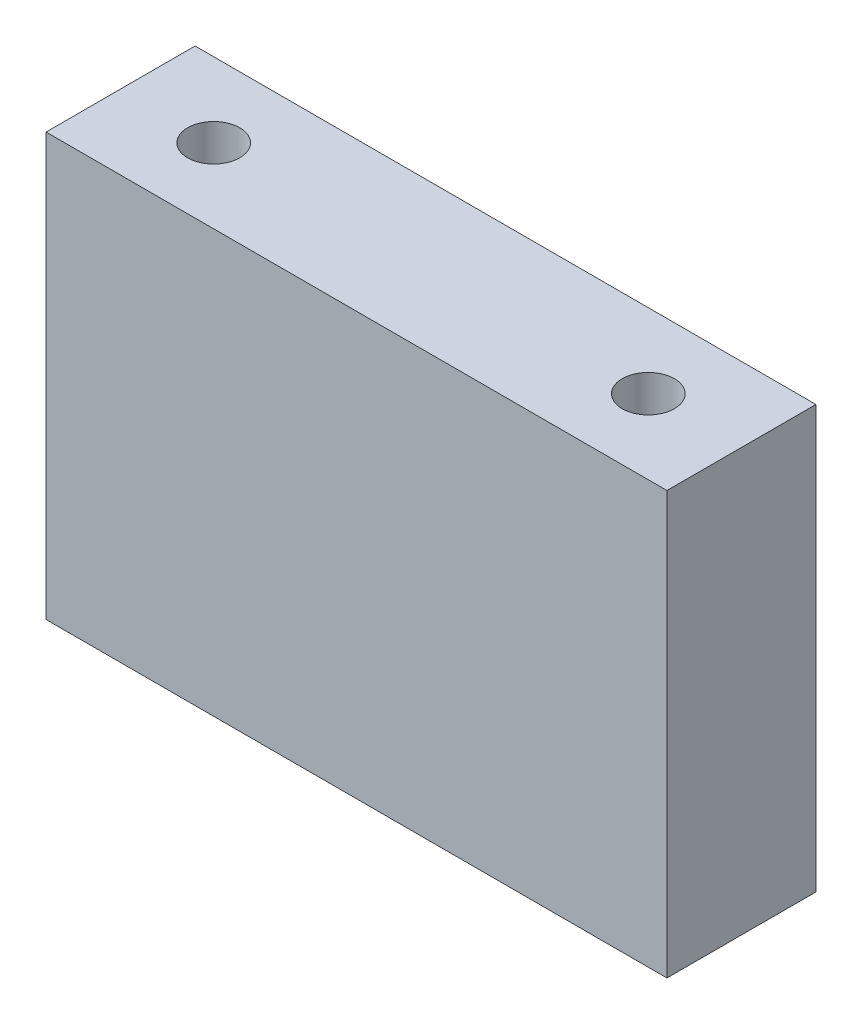
from build123d import *

# Parameters (mm, degrees)
SKETCH_1_W                  = 50
SKETCH_1_H                  = 34
EXTRUDE_1_DEPTH             = 6
HOLE_WIZARD_M5_1_AT_2_COUNT = 2
HOLE_WIZARD_M5_1_AT_2_PITCH = 35


with BuildPart() as part:
    # 草图1 → 凸台-拉伸1 (new, symmetric)
    with BuildSketch(Plane.XY):
        Rectangle(SKETCH_1_W, SKETCH_1_H)
    extrude(amount=EXTRUDE_1_DEPTH, both=True)

    # 草图3 → M5 螺纹孔1 (revolve, cut)
    with BuildSketch(Plane(origin=(-17.5, -17, 0), x_dir=(0, 0, -1), z_dir=(1, 0, 0))):
        Polygon((0, 0), (0, 13.6618073), (2.1, 12.4), (2.1, 0), align=None)
    hole_wizard_m5_1 = revolve(axis=Axis((-17.5, -23.35, 0), (0, 1, 0)), mode=Mode.SUBTRACT)

    # M5 螺纹孔1 at 2: M5 螺纹孔1 ×2
    with Locations(*[(i * HOLE_WIZARD_M5_1_AT_2_PITCH, 0, 0) for i in range(1, HOLE_WIZARD_M5_1_AT_2_COUNT)]):
        add(hole_wizard_m5_1, mode=Mode.SUBTRACT)

    # 镜向1: M5 螺纹孔1 across plane
    add(hole_wizard_m5_1.mirror(Plane.ZX), mode=Mode.SUBTRACT)

    # 镜向1 copy 1 sketch → 镜向1 copy 1 (revolve, cut)
    with BuildSketch(Plane(origin=(17.5, 17, 0), x_dir=(0, 0, -1), z_dir=(1, 0, 0))):
        Polygon((0, 0), (0, -13.6618073), (2.1, -12.4), (2.1, 0), align=None)
    revolve(axis=Axis((17.5, 23.35, 0), (0, 1, 0)), mode=Mode.SUBTRACT)


solid = part.part
